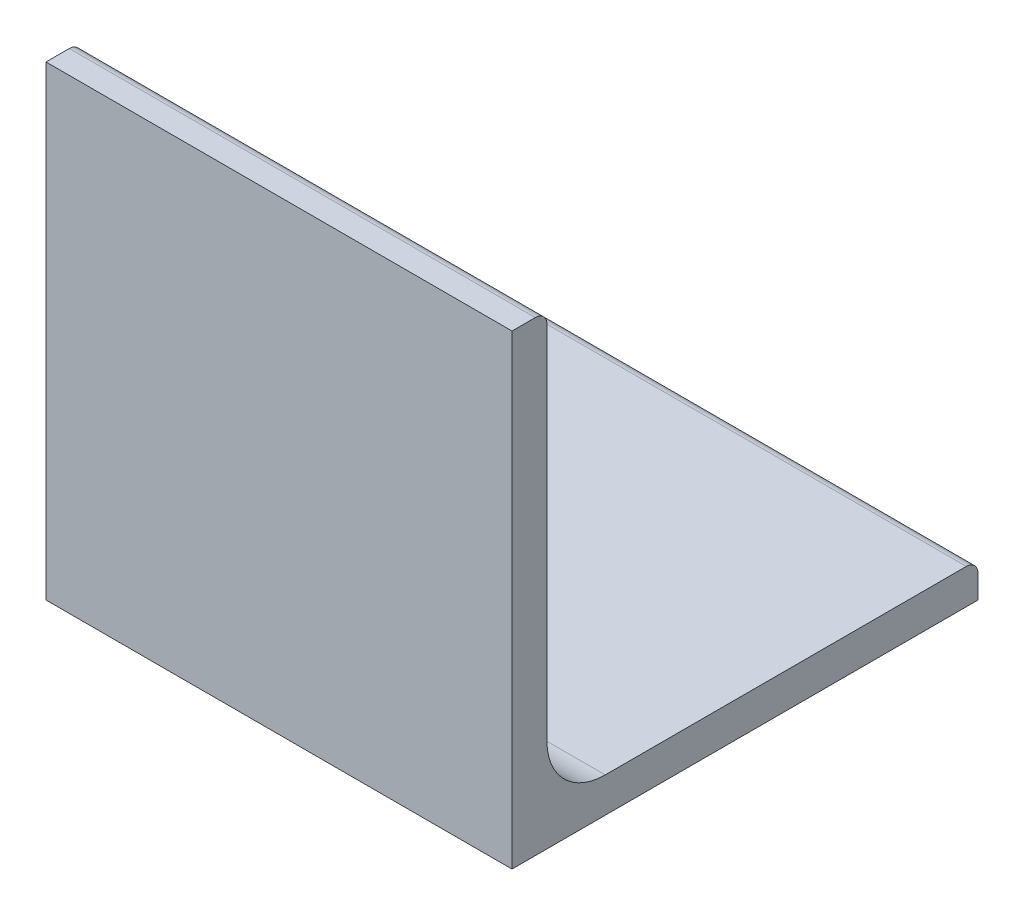
SolidWorks part; units mm, degrees
material "普通碳钢"
ref_plane "前视基准面" through (0, 0, 0) normal (0, 0, 1) x (1, 0, 0)
ref_plane "上视基准面" through (0, 0, 0) normal (0, 1, 0) x (1, 0, 0)
ref_plane "右视基准面" through (0, 0, 0) normal (1, 0, 0) x (0, 0, -1)
sketch3d "3D草图1"
  line L0 (0, 0, 0) -> (40, 0, 0)
  dimension "D1" = 40
other "角铁 40 X 3(1)"
ref_plane "基准面1" through (0, 0, 0) normal (1, 0, 0) x (0, 0, -1)
sketch "Sketch1" plane through (0, 0, 0) normal (1, 0, 0) x (0, 0, -1)
  line L0 (0, 0) -> (0, 40)
  line L1 (0, 20) -> (3, 20) construction
  line L2 (3, 39) -> (3, 8)
  line L3 (8, 3) -> (39, 3)
  line L4 (20, 3) -> (20, 0) construction
  line L5 (40, 0) -> (0, 0)
  line L6 (0, 40) -> (2, 40)
  line L7 (40, 0) -> (40, 2)
  arc A0 (40, 2) -> (39, 3) centre (39, 2) ccw
  arc A1 (2, 40) -> (3, 39) centre (2, 39) cw
  arc A2 (8, 3) -> (3, 8) centre (8, 8) cw
  point P10 (20, 0)
  point P14 (0, 20)
  point P15 (3, 20)
  point P16 (20, 3)
  point P17 (3, 40)
  point P18 (40, 3)
  point P21 (40, 3)
  point P24 (3, 40)
  point P25 (0, 0)
equation "\"D2@Sketch1\" = \"D1@Sketch1\" / 3"
